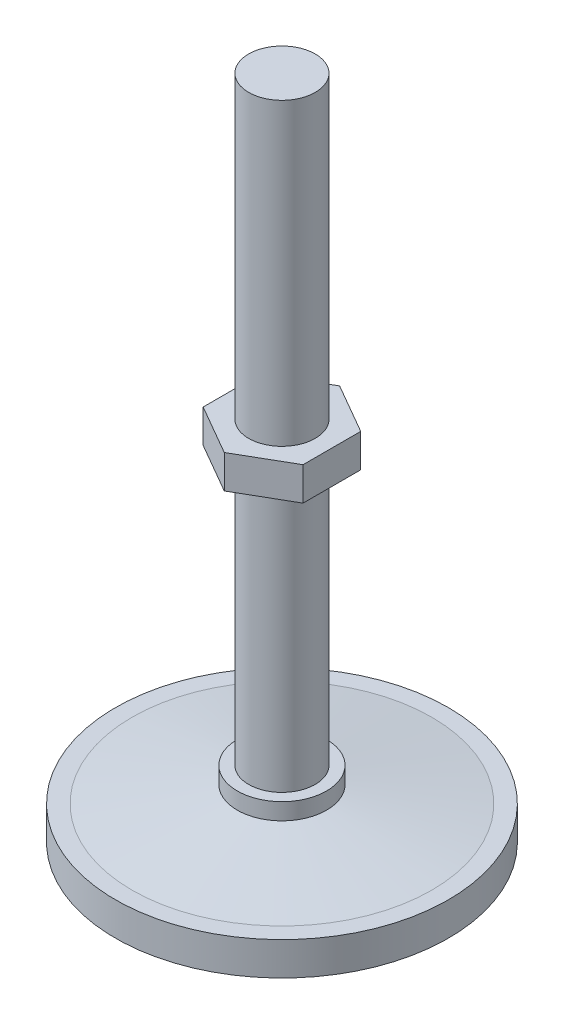
SolidWorks part; units mm, degrees
ref_plane "Front Plane" through (0, 0, 0) normal (0, 0, 1) x (1, 0, 0)
ref_plane "Top Plane" through (0, 0, 0) normal (0, 1, 0) x (1, 0, 0)
ref_plane "Right Plane" through (0, 0, 0) normal (1, 0, 0) x (0, 0, -1)
sketch "Sketch1" plane through (0, 0, 0) normal (0, 0, 1) x (1, 0, 0)
  line L0 (0, 0) -> (0, 231.4656) construction
  line L1 (0, 0) -> (50, 0)
  line L2 (50, 0) -> (50, 10)
  line L3 (50, 10) -> (45, 10)
  line L4 (45, 10) -> (13.4046, 15)
  line L5 (13.4046, 15) -> (13.4046, 20)
  line L6 (13.4046, 20) -> (10, 20)
  line L7 (10, 20) -> (10, 200)
  line L8 (10, 200) -> (0, 200)
  line L9 (0, 200) -> (0, 0)
  dimension "D1" = 20
  dimension "D2" = 200
  dimension "D3" = 10
  dimension "D4" = 5
  dimension "D5" = 5
  dimension "D6" = 20
  dimension "D7" = 100
revolve "Revolve1" add sketch "Sketch1" angle 360 about L0
ref_plane "Plane1" through (0, 110, 0) normal (0, -1, 0) x (1, 0, 0)
sketch "Sketch2" plane through (0, 110, 0) normal (0, -1, 0) x (1, 0, 0)
  line L1 (0, 17.3205) -> (-15, 8.6603)
  line L2 (-15, 8.6603) -> (-15, -8.6603)
  line L3 (-15, -8.6603) -> (0, -17.3205)
  line L4 (0, -17.3205) -> (15, -8.6603)
  line L5 (15, -8.6603) -> (15, 8.6603)
  line L6 (15, 8.6603) -> (0, 17.3205)
  circle A0 centre (0, 0) radius 15 construction
  dimension "D1" = 30
extrude "Extrude1" add sketch "Sketch2" along normal blind 10
